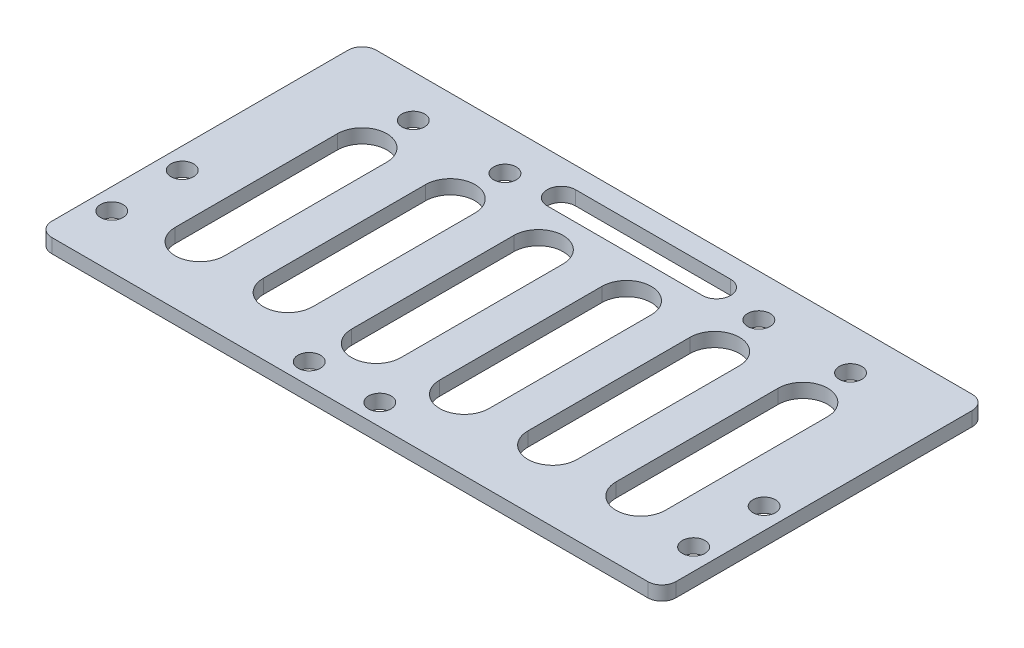
from build123d import *

# Parameters (mm, degrees)
SKETCH_1_W          = 88.5
SKETCH_1_H          = 46
SKETCH_1_R          = 1.6
EXTRUDE_1_DEPTH     = 2
CUT_EXTRUDE_1_DEPTH = 50.910544978
FILLET_1_R          = 2


with BuildPart() as part:
    # 草图1 → 凸台-拉伸1 (new body)
    with BuildSketch(Plane(origin=(0, 0, 0), x_dir=(1, 0, 0), z_dir=(0, 1, 0))):
        Rectangle(SKETCH_1_W, SKETCH_1_H)
        with Locations(Location((-41.25, -5.5, 0), (0, 0, 270))):
            Circle(SKETCH_1_R, mode=Mode.SUBTRACT)
        with Locations(Location((-41.25, -15.5, 0), (0, 0, 270))):
            Circle(SKETCH_1_R, mode=Mode.SUBTRACT)
        with Locations(Location((41.25, -15.5, 0), (0, 0, 90))):
            Circle(SKETCH_1_R, mode=Mode.SUBTRACT)
        with Locations(Location((41.25, -5.5, 0), (0, 0, 90))):
            Circle(SKETCH_1_R, mode=Mode.SUBTRACT)
        with Locations(Location((-8.75, -20, 0), (0, 0, 270))):
            Circle(SKETCH_1_R, mode=Mode.SUBTRACT)
        with Locations(Location((1.25, -20, 0), (0, 0, 270))):
            Circle(SKETCH_1_R, mode=Mode.SUBTRACT)
        with Locations(Location((-31, 17, 0), (0, 0, 270))):
            Circle(SKETCH_1_R, mode=Mode.SUBTRACT)
        with Locations(Location((-18, 17, 0), (0, 0, 270))):
            Circle(SKETCH_1_R, mode=Mode.SUBTRACT)
        with Locations(Location((18, 17, 0), (0, 0, 270))):
            Circle(SKETCH_1_R, mode=Mode.SUBTRACT)
        with Locations(Location((31, 17, 0), (0, 0, 270))):
            Circle(SKETCH_1_R, mode=Mode.SUBTRACT)
    extrude(amount=EXTRUDE_1_DEPTH)

    # 草图2 → 切除-拉伸1 (cut, through all)
    with BuildSketch(Plane(origin=(0, 2, 0), x_dir=(1, 0, 0), z_dir=(0, 1, 0))):
        with BuildLine():
            Line((-27.75, 10), (-27.75, -13))
            ThreePointArc((-27.75, -13), (-31.25, -16.5), (-34.75, -13))
            Line((-34.75, -13), (-34.75, 10))
            ThreePointArc((-34.75, 10), (-31.25, 13.5), (-27.75, 10))
        make_face()
        with BuildLine():
            Line((-15.25, 10), (-15.25, -13))
            ThreePointArc((-15.25, -13), (-18.75, -16.5), (-22.25, -13))
            Line((-22.25, -13), (-22.25, 10))
            ThreePointArc((-22.25, 10), (-18.75, 13.5), (-15.25, 10))
        make_face()
        with BuildLine():
            Line((-2.75, 10), (-2.75, -13))
            ThreePointArc((-2.75, -13), (-6.25, -16.5), (-9.75, -13))
            Line((-9.75, -13), (-9.75, 10))
            ThreePointArc((-9.75, 10), (-6.25, 13.5), (-2.75, 10))
        make_face()
        with BuildLine():
            Line((9.75, 10), (9.75, -13))
            ThreePointArc((9.75, -13), (6.25, -16.5), (2.75, -13))
            Line((2.75, -13), (2.75, 10))
            ThreePointArc((2.75, 10), (6.25, 13.5), (9.75, 10))
        make_face()
        with BuildLine():
            Line((22.25, 10), (22.25, -13))
            ThreePointArc((22.25, -13), (18.75, -16.5), (15.25, -13))
            Line((15.25, -13), (15.25, 10))
            ThreePointArc((15.25, 10), (18.75, 13.5), (22.25, 10))
        make_face()
        with BuildLine():
            Line((34.75, 10), (34.75, -13))
            ThreePointArc((34.75, -13), (31.25, -16.5), (27.75, -13))
            Line((27.75, -13), (27.75, 10))
            ThreePointArc((27.75, 10), (31.25, 13.5), (34.75, 10))
        make_face()
        with BuildLine():
            Line((-11, 20), (11, 20))
            ThreePointArc((11, 20), (13, 18), (11, 16))
            Line((11, 16), (-11, 16))
            ThreePointArc((-11, 16), (-13, 18), (-11, 20))
        make_face()
    extrude(amount=-CUT_EXTRUDE_1_DEPTH, mode=Mode.SUBTRACT)

    # 圆角1
    fillet_1_edges = [part.edges().sort_by_distance(p)[0] for p in [
        (44.25, 1, 23),
        (-44.25, 1, 23),
        (-44.25, 1, -23),
        (44.25, 1, -23),
    ]]
    fillet(fillet_1_edges, radius=FILLET_1_R)


solid = part.part
